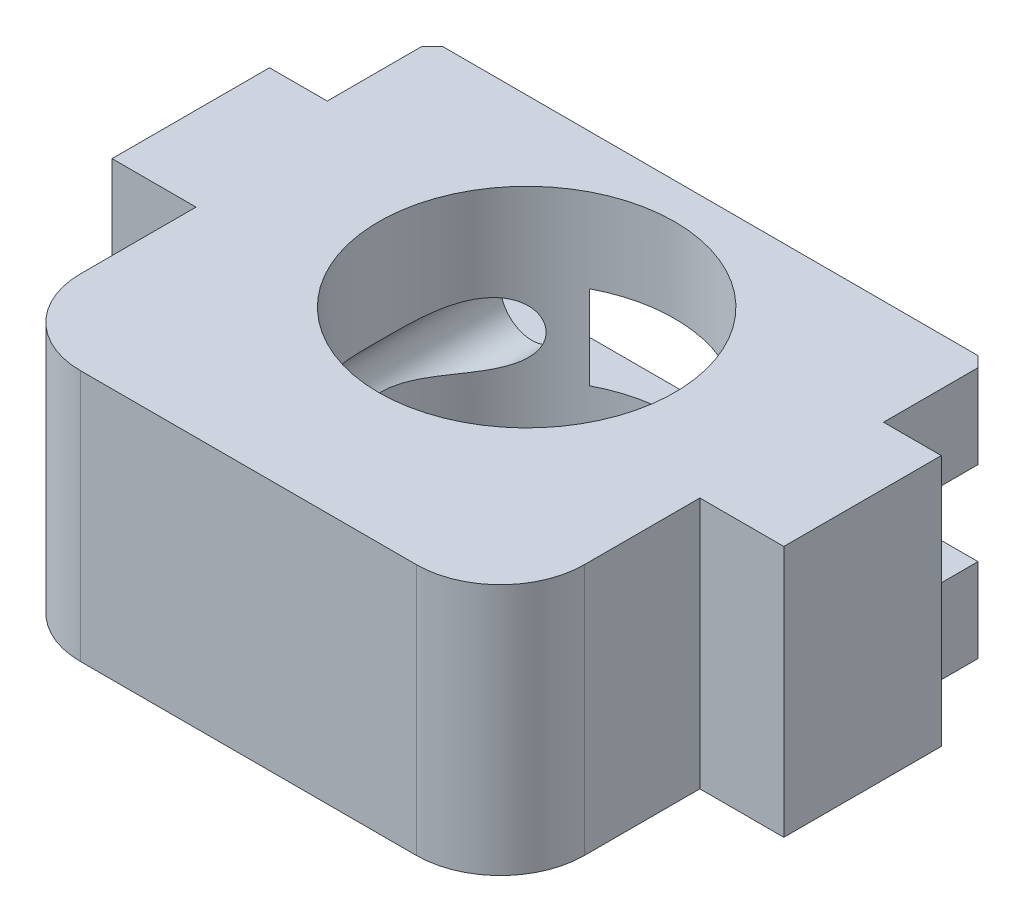
SolidWorks part; units mm, degrees
ref_plane "Front Plane" through (0, 0, 0) normal (0, 0, 1) x (1, 0, 0)
ref_plane "Top Plane" through (0, 0, 0) normal (0, 1, 0) x (1, 0, 0)
ref_plane "Right Plane" through (0, 0, 0) normal (1, 0, 0) x (0, 0, -1)
sketch "Sketch1" plane through (0, 0, 0) normal (0, 1, 0) x (1, 0, 0)
  line L0 (0, 38.2466) -> (0, -42.6214) construction
  line L1 (-24, 19) -> (-24, 8)
  line L2 (-24, 19) -> (-32, 19)
  line L3 (-32, 19) -> (-32, 34)
  line L4 (-32, 34) -> (-26.5, 34)
  line L5 (-26.5, 34) -> (-26.5, 44)
  line L6 (-26.5, 44) -> (26.5, 44)
  line L7 (-16, 0) -> (16, 0)
  line L8 (26.5, 34) -> (26.5, 44)
  line L9 (32, 34) -> (26.5, 34)
  line L10 (32, 19) -> (32, 34)
  line L11 (24, 19) -> (32, 19)
  line L12 (24, 19) -> (24, 8)
  arc A0 (-24, 8) -> (-16, 0) centre (-16, 8) ccw
  arc A1 (24, 8) -> (16, 0) centre (16, 8) cw
  point P14 (0, 0)
  dimension "D4" = 8
  dimension "D1" = 53
  dimension "D2" = 64
  dimension "D3" = 48
  dimension "D5" = 10
  dimension "D6" = 15
  dimension "D7" = 44
extrude "Boss-Extrude1" add sketch "Sketch1" along normal blind 24
sketch "Sketch2" plane through (-26.5, 0, 0) normal (-1, 0, 0) x (0, 0, 1)
  line L0 (-44, 24) -> (-44, 0) construction
  line L1 (-44, 16) -> (-39, 16)
  line L2 (-44, 16) -> (-44, 8)
  line L3 (-44, 8) -> (-39, 8)
  line L4 (-39, 16) -> (-39, 8)
  line L5 (-44, 16) -> (-39, 8) construction
  line L6 (-44, 8) -> (-39, 16) construction
  line L7 (-44, 24) -> (-34, 24) construction
  point P0 (-44, 12)
  point P10 (-44, 12)
  dimension "D1" = 5
  dimension "D2" = 8
  dimension "D3" = 12
extrude "Cut-Extrude1" cut sketch "Sketch2" against normal blind 64
sketch "Sketch3" plane through (0, 0, -39) normal (0, 0, -1) x (-1, 0, 0)
  line L0 (-32, 12) -> (32, 12) construction
  line L1 (-32, 24) -> (-32, 0) construction
  line L2 (32, 24) -> (32, 0) construction
  line L4 (0, 24) -> (0, -3.6148) construction
  line L5 (-26.5, 24) -> (26.5, 24) construction
  circle A0 centre (-12, 12) radius 3
  circle A1 centre (12, 12) radius 3
  dimension "D1" = 6
  dimension "D2" = 24
extrude "Cut-Extrude2" cut sketch "Sketch3" against normal blind 35
sketch "Sketch4" plane through (0, 0, 0) normal (0, -1, 0) x (1, 0, 0)
  circle A0 centre (0, -26.5) radius 14.1
  dimension "D1" = 28.2
extrude "Cut-Extrude3" cut sketch "Sketch4" against normal blind 35
chamfer "Chamfer1" distance 1 angle 45 6 edges at (26.5, 4, -44) (0, 8, -44) (-26.5, 4, -44) (26.5, 20, -44) (0, 16, -44) (-26.5, 20, -44)
chamfer "Chamfer2" distance 3 angle 45 1 edges at (0, 0, -40.6)
